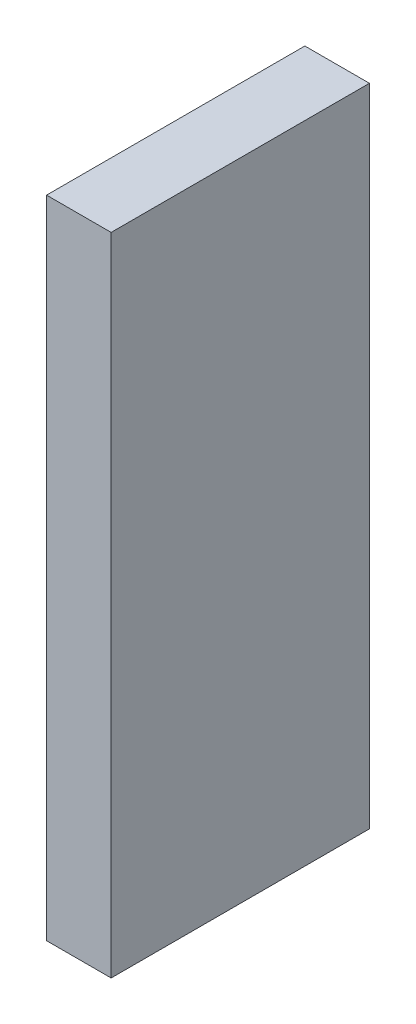
SolidWorks part; units mm, degrees
ref_plane "Front Plane" through (0, 0, 0) normal (0, 0, 1) x (1, 0, 0)
ref_plane "Top Plane" through (0, 0, 0) normal (0, 1, 0) x (1, 0, 0)
ref_plane "Right Plane" through (0, 0, 0) normal (1, 0, 0) x (0, 0, -1)
sketch "Sketch1" plane through (0, 0, 0) normal (0, 0, 1) x (1, 0, 0)
  line L1 (0, 0) -> (25, 0)
  line L2 (0, 0) -> (0, -250)
  line L3 (0, -250) -> (25, -250)
  line L4 (25, 0) -> (25, -250)
  dimension "D1" = 25
  dimension "D2" = 250
extrude "Boss-Extrude1" add sketch "Sketch1" along normal blind 100
